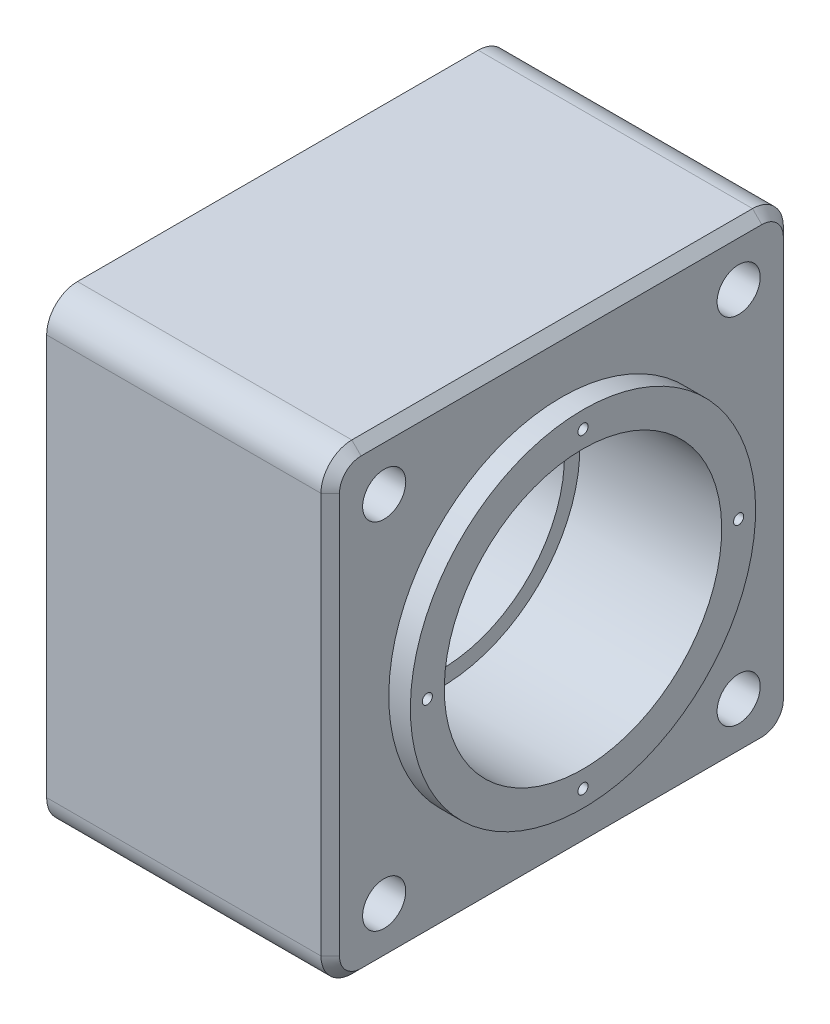
from build123d import *
from build123d.topology import SkipClean

# Parameters (mm, degrees)
SKETCH1_W               = 150
SKETCH1_H               = 150
BOSS_EXTRUDE1_DEPTH     = 92
SKETCH2_R               = 56
BOSS_EXTRUDE2_DEPTH     = 10
SKETCH3_R               = 45
CUT_EXTRUDE1_DEPTH      = 76
SKETCH4_R               = 38.5
CUT_EXTRUDE2_DEPTH      = 49
M10_TAPPED_HOLE1_D      = 8.5
M10_TAPPED_HOLE1_DEPTH  = 24.5
M10_TAPPED_HOLE1_TIP    = 2.553657631
M16_TAPPED_HOLE1_D      = 14
M16_TAPPED_HOLE1_DEPTH  = 35
M16_TAPPED_HOLE1_TIP    = 4.206024333
SKETCH14_R              = 55
CUT_EXTRUDE5_DEPTH      = 3
CHAMFER2_SIZE           = 0.5
SKETCH23_R              = 51.5
SKETCH23_R_2            = 41.5
CUT_EXTRUDE9_DEPTH      = 3
CIRPATTERN1_COUNT       = 4
FILLET1_R               = 10
CHAMFER6_SIZE           = 3
SKETCH30_R              = 2.5
CUT_EXTRUDE12_DEPTH     = 12
G1_8_TAPPED_HOLE1_D     = 8.8
G1_8_TAPPED_HOLE1_DEPTH = 30
G1_8_TAPPED_HOLE1_TIP   = 2.643786724
SKETCH34_R              = 11
CUT_EXTRUDE14_DEPTH     = 3
SKETCH35_R              = 60
CUT_EXTRUDE15_DEPTH     = 10
SKETCH36_R              = 55
SKETCH36_R_2            = 38.5
BOSS_EXTRUDE3_DEPTH     = 3
SKETCH37_R              = 95.296679702
CUT_EXTRUDE16_DEPTH     = 3
BOSS_EXTRUDE4_START     = -61
SKETCH38_R              = 45
SKETCH38_R_2            = 40
BOSS_EXTRUDE4_DEPTH     = 15
CUT_EXTRUDE17_START     = -23
SKETCH39_R              = 45
CUT_EXTRUDE17_DEPTH     = 23
CUT_EXTRUDE18_REACH     = 194.445
SKETCH40_R              = 4.4


with BuildPart() as part:
    # Sketch1 → Boss-Extrude1 (new body)
    with BuildSketch(Plane(origin=(0, 0, 0), x_dir=(0, -1, 0), z_dir=(1, 0, 0))):
        Rectangle(SKETCH1_W, SKETCH1_H)
    extrude(amount=BOSS_EXTRUDE1_DEPTH)

    # Sketch2 → Boss-Extrude2 (add)
    with BuildSketch(Plane(origin=(92, 0, 0), x_dir=(0, -1, 0), z_dir=(1, 0, 0))):
        with Locations(Location((0, 0, 0), (0, 0, 180))):
            Circle(SKETCH2_R)
    extrude(amount=BOSS_EXTRUDE2_DEPTH)

    # Sketch3 → Cut-Extrude1 (cut)
    with BuildSketch(Plane(origin=(0, 0, 0), x_dir=(0, -1, 0), z_dir=(-1, 0, 0))):
        Circle(SKETCH3_R)
    extrude(amount=-CUT_EXTRUDE1_DEPTH, mode=Mode.SUBTRACT)

    # Sketch4 → Cut-Extrude2 (cut)
    with BuildSketch(Plane(origin=(102, 0, 0), x_dir=(0, -1, 0), z_dir=(1, 0, 0))):
        with Locations(Location((0, 0, 0), (0, 0, 180))):
            Circle(SKETCH4_R)
    extrude(amount=-CUT_EXTRUDE2_DEPTH, mode=Mode.SUBTRACT)

    # M10 Tapped Hole1
    with Locations(Plane(origin=(0, 0, 0), x_dir=(0, 1, 0), z_dir=(-1, 0, 0))):
        with Locations((-35, 60), (35, 60), (60, 35), (60, -35), (35, -60), (-35, -60), (-60, -35), (-60, 35)):
            Hole(M10_TAPPED_HOLE1_D / 2, depth=M10_TAPPED_HOLE1_DEPTH)
            with Locations((0, 0, -(M10_TAPPED_HOLE1_DEPTH + M10_TAPPED_HOLE1_TIP / 2))):  # 118° drill point
                Cone(0, M10_TAPPED_HOLE1_D / 2, M10_TAPPED_HOLE1_TIP, mode=Mode.SUBTRACT)

    # M16 Tapped Hole1
    with Locations(Plane(origin=(92, 0, 0), x_dir=(0, -1, 0), z_dir=(1, 0, 0))):
        with Locations((57.5, 57.5), (-57.5, 57.5), (-57.5, -57.5), (57.5, -57.5)):
            Hole(M16_TAPPED_HOLE1_D / 2, depth=M16_TAPPED_HOLE1_DEPTH)
            with Locations((0, 0, -(M16_TAPPED_HOLE1_DEPTH + M16_TAPPED_HOLE1_TIP / 2))):  # 118° drill point
                Cone(0, M16_TAPPED_HOLE1_D / 2, M16_TAPPED_HOLE1_TIP, mode=Mode.SUBTRACT)

    # Sketch14 → Cut-Extrude5 (cut)
    with BuildSketch(Plane(origin=(76, 0, 0), x_dir=(0, -1, 0), z_dir=(-1, 0, 0))):
        Circle(SKETCH14_R)
    extrude(amount=-CUT_EXTRUDE5_DEPTH, mode=Mode.SUBTRACT)

    # Chamfer2
    chamfer2_edges = [part.edges().sort_by_distance(p)[0] for p in [
        (102, -56, 0),
    ]]
    chamfer(chamfer2_edges, length=CHAMFER2_SIZE)

    # Sketch23 → Cut-Extrude9 (cut)
    with BuildSketch(Plane(origin=(102, 0, 0), x_dir=(0, 0, -1), z_dir=(1, 0, 0))):
        with Locations(Location((0, 0, 0), (0, 0, 90))):
            Circle(SKETCH23_R)
        with Locations(Location((0, 0, 0), (0, 0, 90))):
            Circle(SKETCH23_R_2, mode=Mode.SUBTRACT)
    extrude(amount=-CUT_EXTRUDE9_DEPTH, mode=Mode.SUBTRACT)

    # Sketch25 → M4 Tapped Hole2 (revolve, cut)
    with BuildSketch(Plane(origin=(99, 50.5, 0), x_dir=(0, 0, -1), z_dir=(0, 1, 0))):
        Polygon((0, 0), (0, 11.091420021), (1.65, 10.1), (1.65, 0), align=None)
    m4_tapped_hole2 = revolve(axis=Axis((105.35, 50.5, 0), (-1, 0, 0)), mode=Mode.SUBTRACT)

    # CirPattern1: M4 Tapped Hole2 ×4 about axis
    cirpattern1_axis = Axis((0, 0, 0), (1, 0, 0))
    for i in range(1, CIRPATTERN1_COUNT):
        add(m4_tapped_hole2.rotate(cirpattern1_axis, i * 360 / CIRPATTERN1_COUNT), mode=Mode.SUBTRACT)

    # Fillet1
    fillet1_edges = [part.edges().sort_by_distance(p)[0] for p in [
        (46, -75, 75),
        (46, 75, 75),
        (46, 75, -75),
        (46, -75, -75),
    ]]
    fillet(fillet1_edges, radius=FILLET1_R)

    # Chamfer6
    chamfer6_edges = [part.edges().sort_by_distance(p)[0] for p in [
        (92, 0, -75),
        (92, -75, 0),
        (92, 75, 0),
        (92, 0, 75),
        (92, 72.071067812, 72.071067812),
        (92, 72.071067812, -72.071067812),
        (92, -72.071067812, 72.071067812),
        (92, -72.071067812, -72.071067812),
    ]]
    chamfer(chamfer6_edges, length=CHAMFER6_SIZE)

    # Sketch30 → Cut-Extrude12 (cut)
    with BuildSketch(Plane.XZ.offset(75)):
        with Locations(Location((45, 0, 0), (0, 0, 270))):
            Circle(SKETCH30_R)
    extrude(amount=-CUT_EXTRUDE12_DEPTH, mode=Mode.SUBTRACT)

    # G1/8 Tapped Hole1
    with Locations(Plane(origin=(0, -75, 0), x_dir=(-1, 0, 0), z_dir=(0, -1, 0))):
        with Locations((-45, 0)):
            Hole(G1_8_TAPPED_HOLE1_D / 2, depth=G1_8_TAPPED_HOLE1_DEPTH)
            with Locations((0, 0, -(G1_8_TAPPED_HOLE1_DEPTH + G1_8_TAPPED_HOLE1_TIP / 2))):  # 118° drill point
                Cone(0, G1_8_TAPPED_HOLE1_D / 2, G1_8_TAPPED_HOLE1_TIP, mode=Mode.SUBTRACT)

    # Sketch34 → Cut-Extrude14 (cut)
    with BuildSketch(Plane.XZ.offset(75)):
        with Locations(Location((45, 0, 0), (0, 0, 270))):
            Circle(SKETCH34_R)
    extrude(amount=-CUT_EXTRUDE14_DEPTH, mode=Mode.SUBTRACT)

    # Sketch35 → Cut-Extrude15 (cut)
    with BuildSketch(Plane.ZY):
        Circle(SKETCH35_R)
    extrude(amount=-CUT_EXTRUDE15_DEPTH, mode=Mode.SUBTRACT)

    # Sketch36 → Boss-Extrude3 (add)
    with BuildSketch(Plane.ZY.offset(-79)):
        Circle(SKETCH36_R)
        with Locations(Location((0, 0, 0), (0, 0, 90))):
            Circle(SKETCH36_R_2, mode=Mode.SUBTRACT)
    extrude(amount=BOSS_EXTRUDE3_DEPTH)

    # Sketch37 → Cut-Extrude16 (cut)
    with BuildSketch(Plane(origin=(102, 0, 0), x_dir=(0, 0, -1), z_dir=(1, 0, 0))):
        Circle(SKETCH37_R)
    extrude(amount=-CUT_EXTRUDE16_DEPTH, mode=Mode.SUBTRACT)

    # Sketch38 → Boss-Extrude4 (add)
    with BuildSketch(Plane(origin=(99, 0, 0), x_dir=(0, 0, -1), z_dir=(1, 0, 0)).offset(BOSS_EXTRUDE4_START)):
        with Locations(Location((0, 0, 0), (0, 0, 180))):
            Circle(SKETCH38_R)
        with Locations(Location((0, 0, 0), (0, 0, 90))):
            Circle(SKETCH38_R_2, mode=Mode.SUBTRACT)
    extrude(amount=BOSS_EXTRUDE4_DEPTH)

    # Sketch39 → Cut-Extrude17 (cut)
    with SkipClean():  # the faces are left unmerged after this step: merging them gives an invalid solid
        with BuildSketch(Plane(origin=(99, 0, 0), x_dir=(0, 0, -1), z_dir=(1, 0, 0)).offset(CUT_EXTRUDE17_START)):
            with Locations(Location((0, 0, 0), (0, 0, 180))):
                Circle(SKETCH39_R)
        extrude(amount=CUT_EXTRUDE17_DEPTH, mode=Mode.SUBTRACT)

    # Sketch40 → Cut-Extrude18 (cut, up to next)
    with BuildSketch(Plane.XZ.offset(72), mode=Mode.PRIVATE) as cut_extrude18_sk1:
        with Locations(Location((45, 0, 0), (0, 0, 270))):
            Circle(SKETCH40_R)
    cut_extrude18_tool1 = extrude(cut_extrude18_sk1.sketch, amount=-CUT_EXTRUDE18_REACH, mode=Mode.PRIVATE) & part.part
    add(cut_extrude18_tool1.solids().sort_by_distance((45, -72, 0))[0], mode=Mode.SUBTRACT)


solid = part.part
